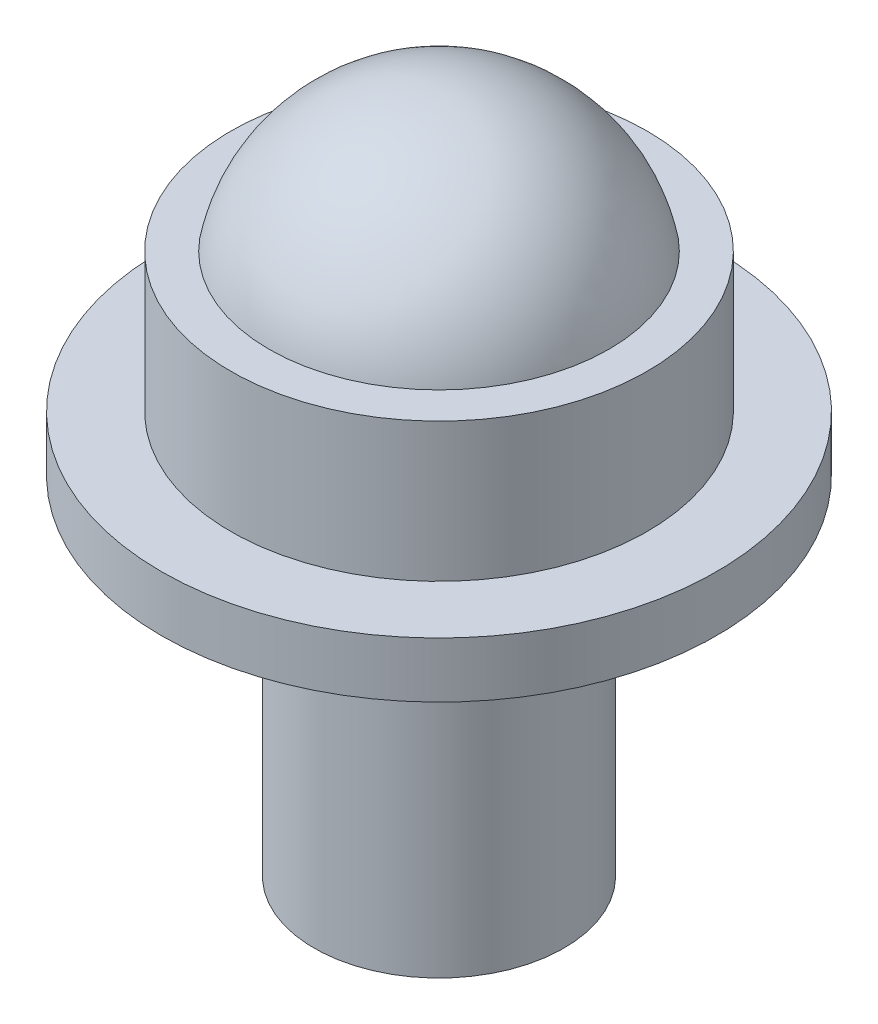
from build123d import *

# Parameters (mm, degrees)
SKETCH2_R           = 18
BOSS_EXTRUDE1_DEPTH = 50


with BuildPart() as part:
    # Sketch1 → Revolve1 (revolve)
    with BuildSketch(Plane.XY, mode=Mode.PRIVATE) as revolve1_sk:
        with BuildLine():
            Line((-24.494897428, 28), (-30, 28))
            Line((-30, 28), (-30, 8))
            Line((-30, 8), (-40, 8))
            Line((-40, 8), (-40, 0))
            Line((-40, 0), (0, 0))
            Line((0, 0), (0, 48))
            ThreePointArc((0, 48), (-15.811388301, 42.364916731), (-24.494897428, 28))
        make_face()
    revolve(revolve1_sk.sketch.rotate(Axis((0, 0, 0), (0, 1, 0)), 270), axis=Axis((0, 0, 0), (0, 1, 0)))

    # Sketch2 → Boss-Extrude1 (add)
    with BuildSketch(Plane(origin=(0, 0, 0), x_dir=(-1, 0, 0), z_dir=(0, -1, 0))):
        with Locations(Location((0, 0, 0), (0, 0, 90))):
            Circle(SKETCH2_R)
    extrude(amount=BOSS_EXTRUDE1_DEPTH)


solid = part.part
